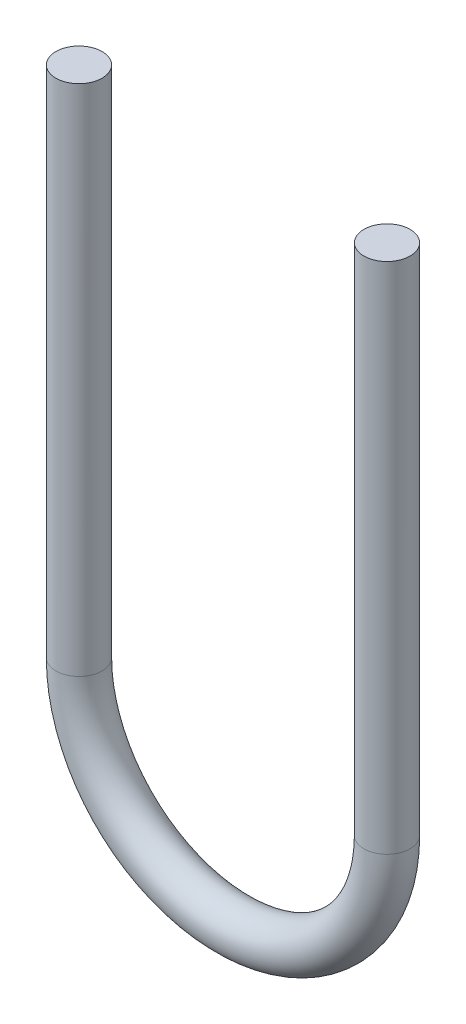
SolidWorks part; units mm, degrees
ref_plane "Front Plane" through (0, 0, 0) normal (0, 0, 1) x (1, 0, 0)
ref_plane "Top Plane" through (0, 0, 0) normal (0, 1, 0) x (1, 0, 0)
ref_plane "Right Plane" through (0, 0, 0) normal (1, 0, 0) x (0, 0, -1)
sketch "Sketch1" plane through (0, 0, 0) normal (0, 0, 1) x (1, 0, 0)
  line L1 (60, 0) -> (60, -100)
  line L2 (0, 0) -> (0, -100)
  arc A1 (0, -100) -> (60, -100) centre (30, -100) ccw
sketch "Sketch2" plane through (0, 0, 0) normal (0, 1, 0) x (1, 0, 0)
  circle A0 centre (0, 0) radius 4.5
  dimension "D1" = 9
sweep "Sweep1" add profiles "Sketch2" path "Sketch1"
